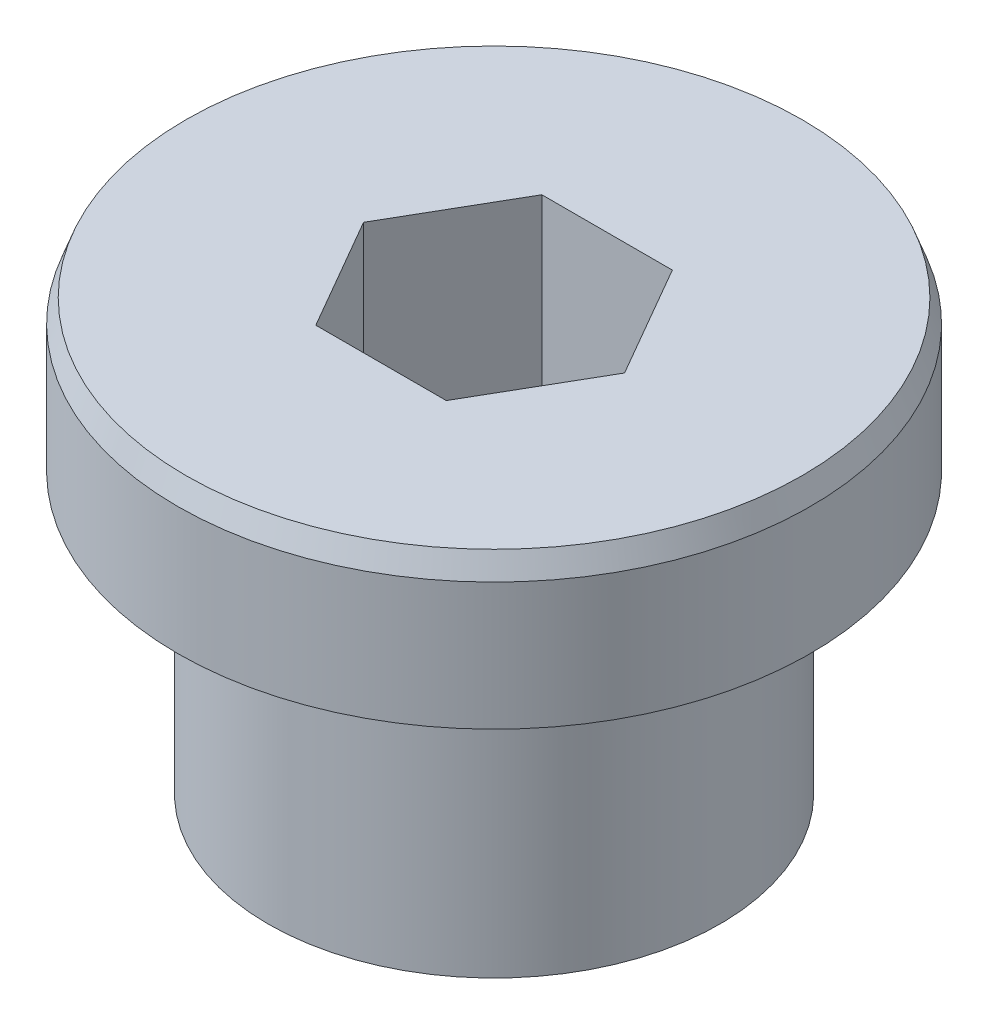
SolidWorks part; units mm, degrees
ref_plane "Front Plane" through (0, 0, 0) normal (0, 0, 1) x (1, 0, 0)
ref_plane "Top Plane" through (0, 0, 0) normal (0, 1, 0) x (1, 0, 0)
ref_plane "Right Plane" through (0, 0, 0) normal (1, 0, 0) x (0, 0, -1)
sketch "Sketch1" plane through (0, 0, 0) normal (0, 1, 0) x (1, 0, 0)
  circle A0 centre (0, 0) radius 5
  dimension "D1" = 10
extrude "Boss-Extrude1" add sketch "Sketch1" along normal blind 6
sketch "Sketch3" plane through (0, 6, 0) normal (0, 1, 0) x (1, 0, 0)
  circle A0 centre (0, 0) radius 7
  dimension "D1" = 14
extrude "Boss-Extrude2" add sketch "Sketch3" along normal blind 3.5
sketch "Sketch4" plane through (0, 9.5, 0) normal (0, 1, 0) x (1, 0, 0)
  line L1 (-2.8868, 0) -> (-1.4434, -2.5)
  line L2 (-1.4434, -2.5) -> (1.4434, -2.5)
  line L3 (1.4434, -2.5) -> (2.8868, 0)
  line L4 (2.8868, 0) -> (1.4434, 2.5)
  line L5 (1.4434, 2.5) -> (-1.4434, 2.5)
  line L6 (-1.4434, 2.5) -> (-2.8868, 0)
  circle A0 centre (0, 0) radius 2.5 construction
  dimension "D1" = 5
extrude "Cut-Extrude1" cut sketch "Sketch4" against normal blind 5
chamfer "Chamfer1" distance 0.5 angle 20 2 edges at (0, 6, 7) (0, 9.5, 7)
